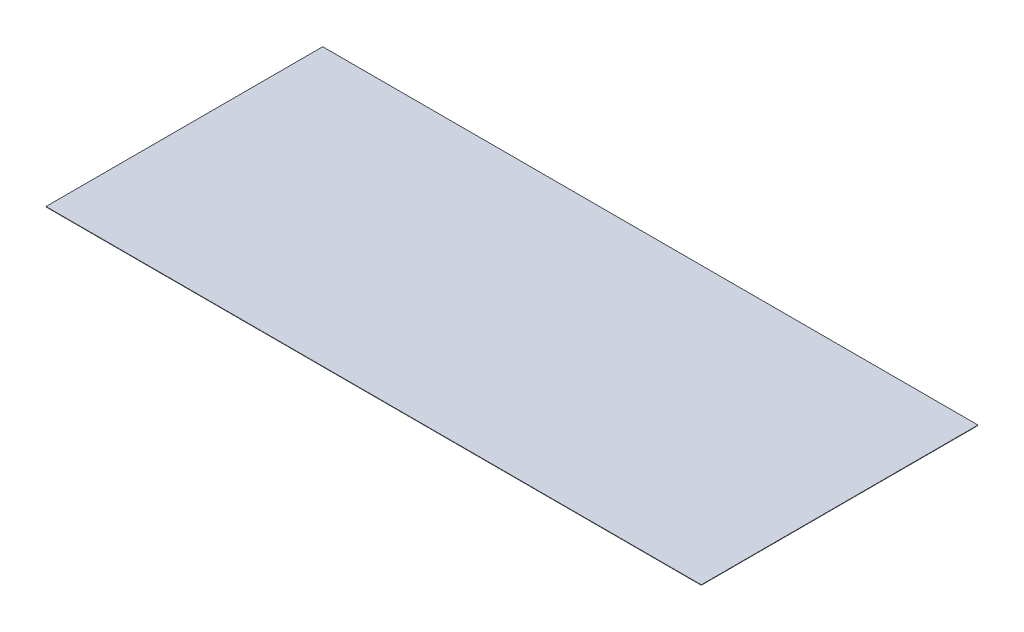
from build123d import *

# Parameters (mm, degrees)
SKETCH_1_W           = 5020
SKETCH_1_H           = 2120
BOSS_EXTRUDE_1_DEPTH = 3


with BuildPart() as part:
    # Sketch 1 → Boss-Extrude 1 (new body)
    with BuildSketch(Plane(origin=(0, 0, 0), x_dir=(1, 0, 0), z_dir=(0, 1, 0))):
        Rectangle(SKETCH_1_W, SKETCH_1_H)
    extrude(amount=BOSS_EXTRUDE_1_DEPTH)


solid = part.part
